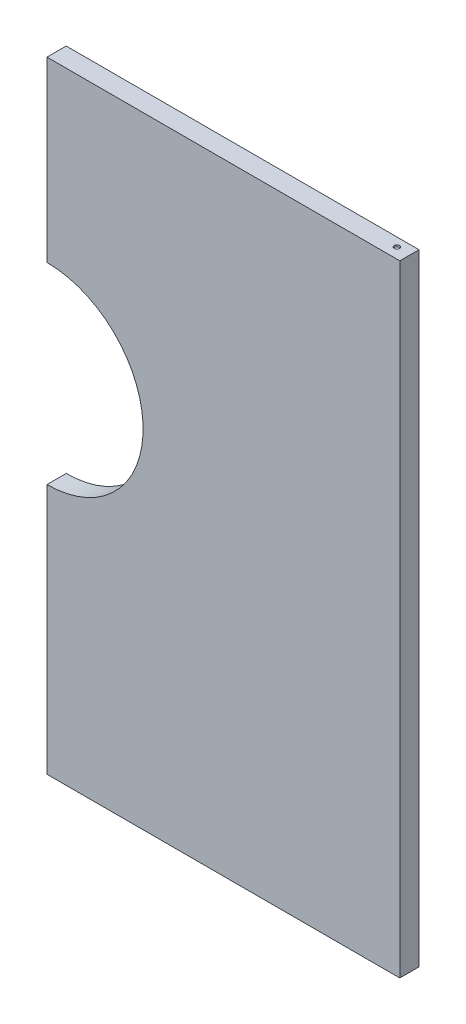
SolidWorks part; units mm, degrees
ref_plane "前视基准面" through (0, 0, 0) normal (0, 0, 1) x (1, 0, 0)
ref_plane "上视基准面" through (0, 0, 0) normal (0, 1, 0) x (1, 0, 0)
ref_plane "右视基准面" through (0, 0, 0) normal (1, 0, 0) x (0, 0, -1)
sketch "草图1" plane through (0, 0, 0) normal (0, 0, 1) x (1, 0, 0)
  line L0 (0, 461) -> (0, 646)
  line L1 (0, 0) -> (367, 0)
  line L2 (0, 0) -> (0, 261)
  line L3 (0, 646) -> (367, 646)
  line L4 (367, 0) -> (367, 646)
  arc A0 (0, 261) -> (0, 461) centre (0, 361) ccw
  dimension "D3" = 285
  dimension "D4" = 200
  dimension "D1" = 646
  dimension "D2" = 367
extrude "凸台-拉伸1" add sketch "草图1" along normal blind 20
shell "抽壳1" thickness 2
sketch "草图2" plane through (0, 2, 0) normal (0, 1, 0) x (1, 0, 0)
  line L0 (365, -9) -> (-62.5815, -9) construction
  line L1 (365, -18) -> (365, 0) construction
  line L3 (367, -20) -> (367, 0) construction
  circle A0 centre (353, -9) radius 2.75
  dimension "D1" = 5.5
  dimension "D2" = 14
extrude "切除-拉伸1" cut sketch "草图2" against normal blind 76 and the other way blind 792
sketch "草图3" plane through (2, 0, 0) normal (1, 0, 0) x (0, 0, -1)
  line L0 (-9, 644) -> (-9, -47.9171) construction
  line L1 (-18, 644) -> (0, 644) construction
  line L2 (-20, 646) -> (0, 646) construction
  line L4 (-20, 0) -> (0, 0) construction
  circle A0 centre (-9, 632) radius 2.75
  circle A1 centre (-9, 552) radius 2.75
  circle A2 centre (-9, 472) radius 2.75
  circle A3 centre (-9, 14) radius 2.75
  circle A4 centre (-9, 129) radius 2.75
  circle A5 centre (-9, 244) radius 2.75
  dimension "D1" = 5.5
  dimension "D2" = 5.5
  dimension "D3" = 5.5
  dimension "D4" = 14
  dimension "D5" = 80
  dimension "D6" = 80
  dimension "D7" = 5.5
  dimension "D8" = 5.5
  dimension "D9" = 5.5
  dimension "D10" = 14
  dimension "D11" = 115
  dimension "D12" = 115
extrude "切除-拉伸2" cut sketch "草图3" against normal blind 10
